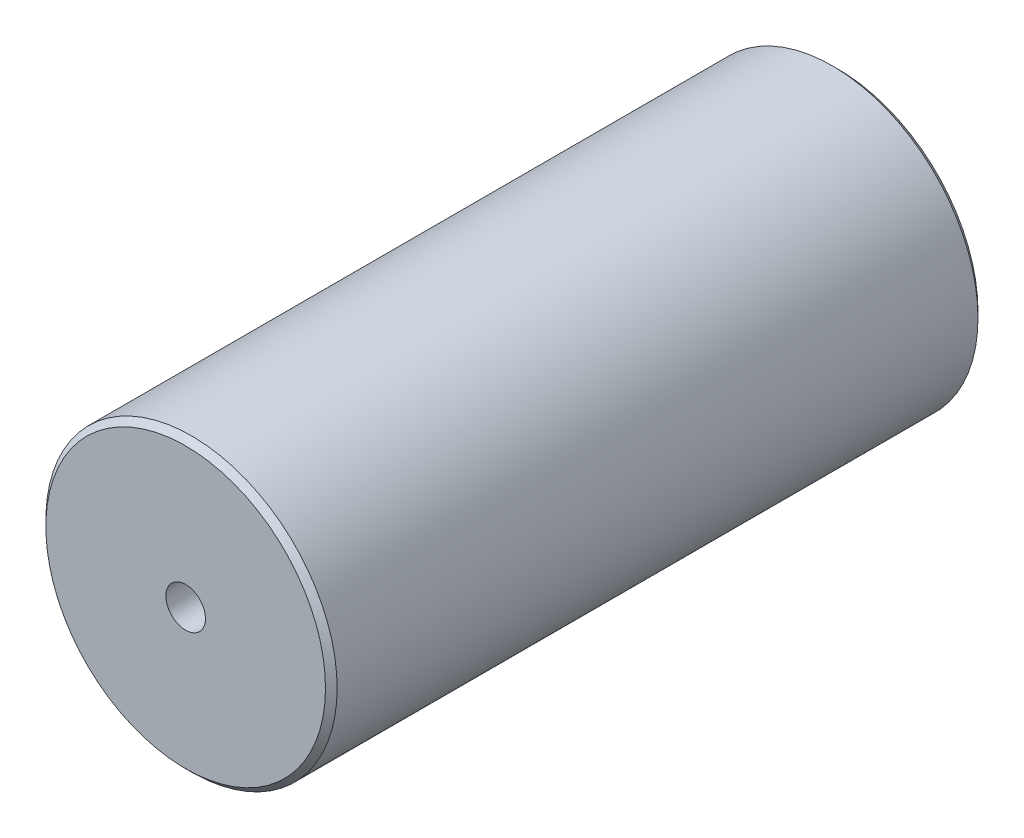
SolidWorks part; units mm, degrees
ref_plane "Front Plane" through (0, 0, 0) normal (0, 0, 1) x (1, 0, 0)
ref_plane "Top Plane" through (0, 0, 0) normal (0, 1, 0) x (1, 0, 0)
ref_plane "Right Plane" through (0, 0, 0) normal (1, 0, 0) x (0, 0, -1)
sketch "Sketch1" plane through (0, 0, 0) normal (0, 0, 1) x (1, 0, 0)
  circle A0 centre (0, 0) radius 25
  dimension "D1" = 50
extrude "Boss-Extrude1" add sketch "Sketch1" along normal blind 112
hole_wizard "M8 Tapped Hole1" positions "Sketch2" profile "Sketch3" tap size "M8" standard "GB"
sketch "Sketch2" plane through (0, 0, 112) normal (0, 0, 1) x (1, 0, 0)
  point P0 (0, 0)
cosmetic thread "Cosmetic Thread1"
sketch "Sketch3" plane through (0, 0, 112) normal (1, 0, 0) x (0, -1, 0)
  line L0 (0, 0) -> (0, 24.0429)
  line L1 (0, 24.0429) -> (3.4, 22)
  line L2 (3.4, 22) -> (3.4, 0)
  line L5 (3.4, 0) -> (0, 0)
  line L10 (0, 24.0429) -> (-3.4, 22) construction
  line L11 (0, -6.35) -> (0, 107.95) construction
  dimension "螺纹孔钻头直径" = 6.8
  dimension "螺纹孔钻头深度" = 22
  dimension "导头角度" = 118
hole_wizard "M8 Tapped Hole2" positions "Sketch4" profile "Sketch5" tap size "M8" standard "GB"
sketch "Sketch4" plane through (0, 0, 0) normal (0, 0, -1) x (-1, 0, 0)
  point P0 (0, 0)
sketch "Sketch5" plane through (0, 0, 0) normal (1, 0, 0) x (0, 1, 0)
  line L0 (0, 0) -> (0, 25.7929)
  line L1 (0, 25.7929) -> (3.4, 23.75)
  line L2 (3.4, 23.75) -> (3.4, 0)
  line L5 (3.4, 0) -> (0, 0)
  line L10 (0, 25.7929) -> (-3.4, 23.75) construction
  line L11 (0, -6.35) -> (0, 107.95) construction
  dimension "螺纹孔钻头直径" = 6.8
  dimension "螺纹孔钻头深度" = 23.75
  dimension "导头角度" = 118
cosmetic thread "Cosmetic Thread2"
chamfer "Chamfer1" distance 1 angle 45 2 edges at (25, 0, 0) (25, 0, 112)
